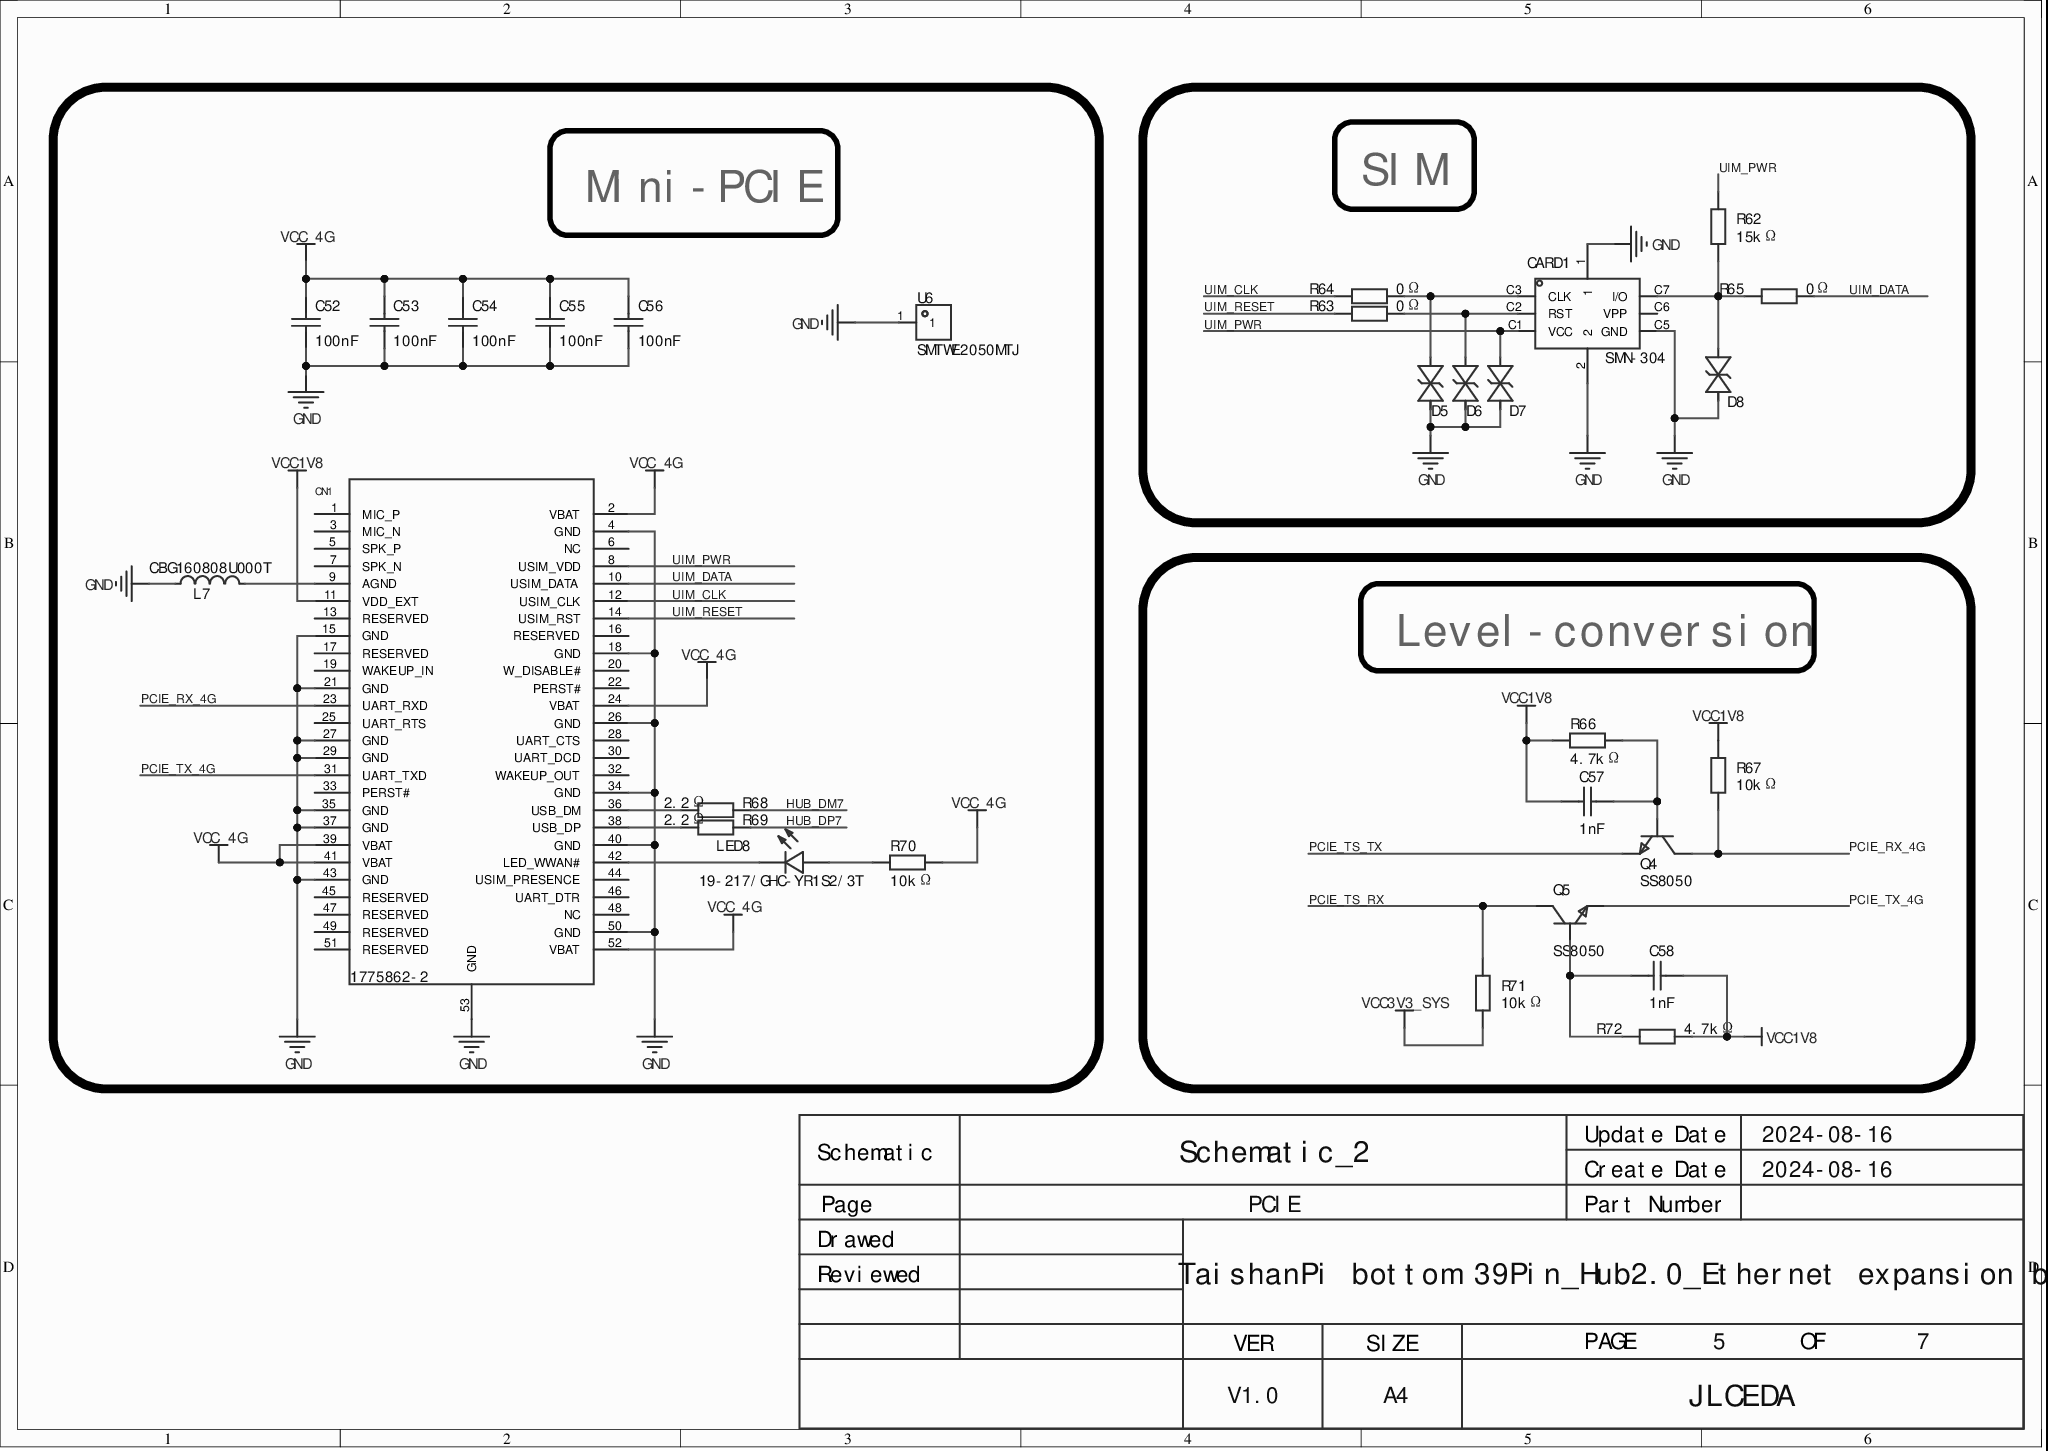
[diagram p0: MISC84334-6.SchDoc]
# Altium project MISC84334.PrjPcb (part 4 of 5)
## Sheet MISC84334-6.SchDoc (continued)
### Library data of the parts (continued)
R70 = 0402WGF1002TCE: Resistor type:Thick film resistor;Resistance:10kΩ;Tolerance:±1%;Power:62.5mW;Max working voltage:50V;Temp. coefficient:±100ppm/℃;; Manufacturer: UNI-ROYAL(厚声); Symbol: RC0402JR-07510RL; AddInBom: yes; ModelId: 671aefced39d4c318694bba8bd8efd39; ModelName: R0402_L1.0-W0.5-H0.5; ModelTransform: 39.37,19.685,0,0,0,0,0,0.0005,0; Tolerance: ±1%; Power(Watts): 62.5mW; Overload Voltage (Max): 50V; LCSC Part Name: 10kΩ ±1% 62.5mW 厚膜电阻; JLCPCB Part Class: Basic Part; Device: 0402WGF1002TCE; SupplierPart: C25744; ManufacturerPart: 0402WGF1002TCE; Supplier Footprint: 0402; Datasheet: https://atta.szlcsc.com/upload/public/pdf/source/20200306/C422600_1E6D84923E4A46A82E41ADD87F860B5C.pdf; Supplier: LCSC; ConvertToPcb: yes; FootprintName: R0402; Type: Thick film resistor; Value: 10kΩ; Temperature Coefficient: ±100ppm/℃; Operating Temperature Range: -55℃~+155℃
U6 = SMTWE2050MTJ: M2x4.35xL5+1.4; Symbol: SMTWE205MTJ; AddInBom: yes; ModelId: 49167c91e1ea4c02a5f8b62a6a5870e0; ModelTransform: 171.2595,171.17147,0,0,0,0,-0.002,0,-55.118; Supplier Part: C2928179; Device: SMTWE2050MTJ; Supplier: LCSC; Manufacturer Part: SMTWE2050MTJ; LCSC Part Name: 雄和远景，电路板表贴圆螺母柱，M2X5，铁镀锡; Supplier Footprint: -; Datasheet: https://atta.szlcsc.com/upload/public/pdf/source/20211223/4247FA230B3B7DF26F2B26B8CCB35E37.pdf; ConvertToPcb: yes; FootprintName: SMD_BD4.4-L4.4-D2.8; ModelName: SMD_BD4.4-L4.4-D2.8

## Sheet MISC84334-7.SchDoc
size 297 x 210 mm; Symbol: Sheet-Symbol_A4; Company: JLCEDA; Version: V1.0; Page Size: A4; @Project Name: TaishanPi bottom 4G_HUB2.0_ET100_HS expansion board; @Page Count: 7; @Update Date: 2024-08-16; @Create Date: 2024-08-16; @Schematic Name: Schematic; @Page No: 1; @Page Name: POWER; Device: Sheet-Symbol_A4; @Board Name: TaishanPi bottom 4G_HUB2.0_ET100_HS expansion board; @Create Time: 14:34:06; @Update Time: 14:34:22
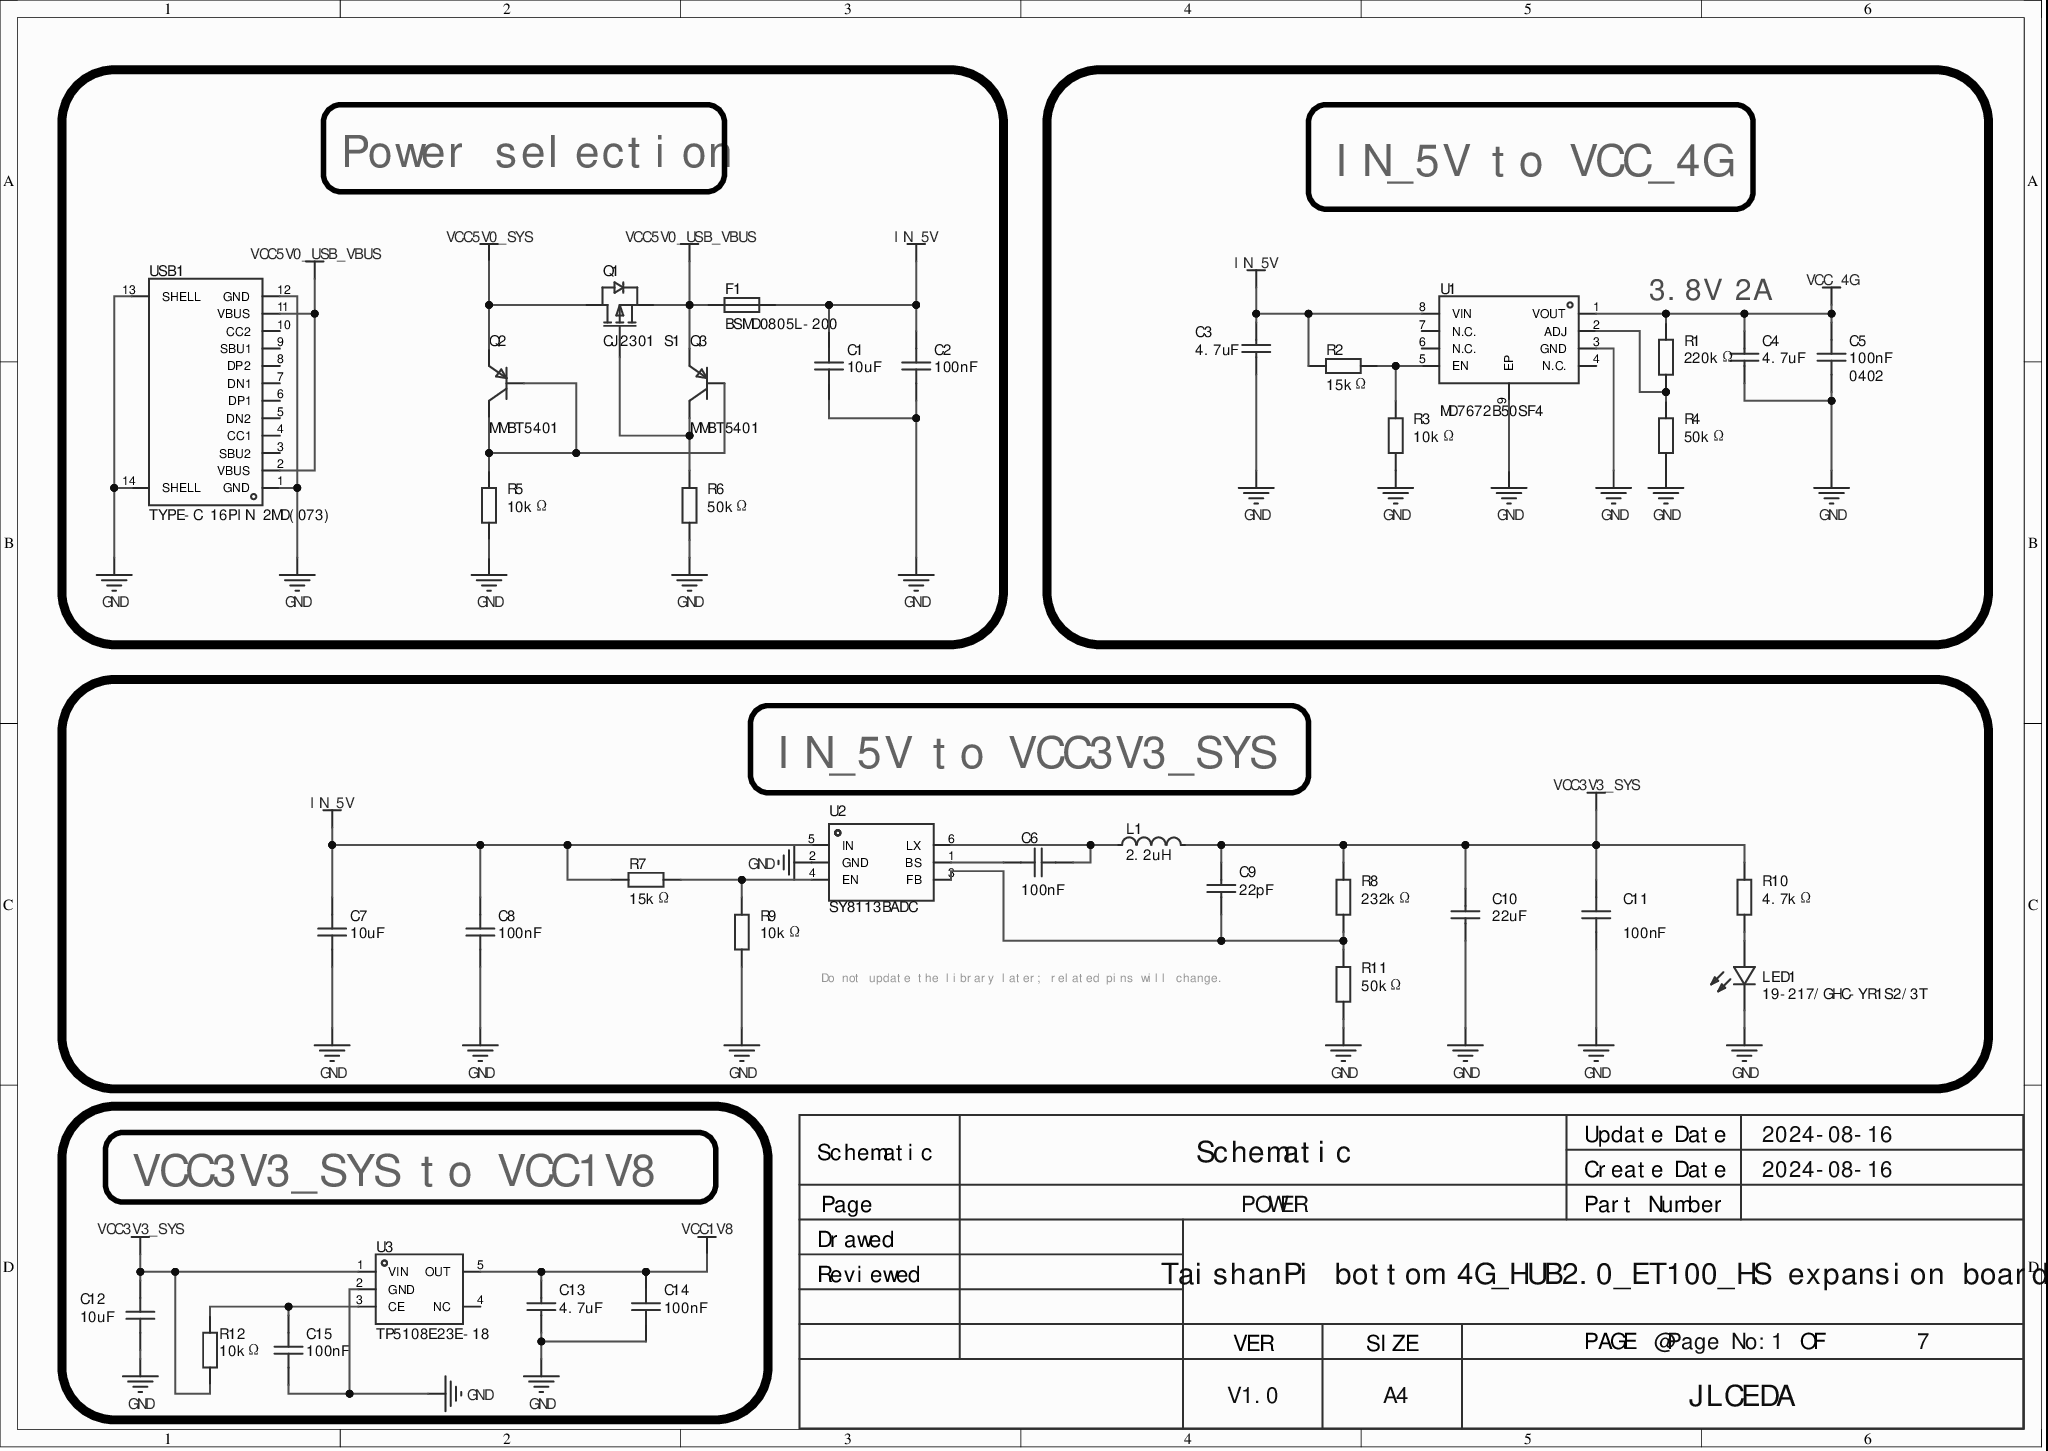
[diagram p1: MISC84334-7.SchDoc]

### Parts
C1  10uF  [r0603]
C2  100nF  [r0603]
C3  4.7uF  [C0603]
C4  4.7uF  [C0603]
C5  100nF  Supplier Footprint: 0402  [R0402]
C6  100nF  [R0402]
C7  10uF  [r0603]
C8  100nF  [r0603]
C9  22pF  [R0402]
C10  22uF  [r0603]
C11  100nF  [r0603]
C12  10uF  [r0603]
C13  4.7uF  [r0603]
C14  100nF  [C0603]
C15  100nF  [C0603]
F1  BSMD0805L-200  [F0805]
L1  2.2uH  [IND-SMD_L2.5-W2.0_WPN252012H]
LED1  19-217/GHC-YR1S2/3T  [LED0603-RD]
Q1  CJ2301 S1  [SOT-23-3_L3.0-W1.7-P0.95-LS2.9-BR]
Q2  MMBT5401  [SOT-23-3_L2.9-W1.3-P1.90-LS2.4-BR]
Q3  MMBT5401  [SOT-23-3_L2.9-W1.3-P1.90-LS2.4-BR]
R1  220kΩ  [R0402]
R2  15kΩ  [R0402]
R3  10kΩ  [R0402]
R4  50kΩ  [R0402]
R5  10kΩ  [R0402]
R6  50kΩ  [R0402]
R7  15kΩ  [R0402]
R8  232kΩ  [R0402]
R9  10kΩ  [R0402]
R10  4.7kΩ  [R0402]
R11  50kΩ  [R0402]
R12  10kΩ  [R0603]
U1  MD7672B50SF4  [ESOP-8_L4.9-W3.9-P1.27-LS6.0-BL-EP]
U2  SY8113BADC  [TSOT-23-6_L2.9-W1.6-P0.95-LS2.8-BR]
U3  TP5108E23E-18  [SOT-23-5_L3.0-W1.7-P0.95-LS2.8-BL]
USB1  TYPE-C 16PIN 2MD(073)  [USB-C-SMD_TYPE-C-6PIN-2MD-073]

### Blocks framed on the sheet
Power selection: C1 C2 F1 Q1-Q3 R5 R6 USB1
IN_5V to VCC_4G: C3-C5 R1-R4 U1
IN_5V to VCC3V3_SYS: C6-C11 L1 LED1 R7-R11 U2
VCC3V3_SYS to VCC1V8: C12-C15 R12 U3

### Nets
GND: C1.1 C2.1 C3.1 C4.1 C5.1 C7.1 C8.1 C10.1 C11.1 C12.1 C13.1 C14.1 C15.1 LED1.1(C) R3.1 R4.1 R5.1 R6.1 R9.1 R11.1 U1.3(GND) U1.9(EP) U2.2(GND) U3.2(GND) USB1.1(GND) USB1.12(GND) USB1.13(SHELL) USB1.14(SHELL)
IN_5V: C1.2 C2.2 C3.2 C7.2 C8.2 F1.2 R2.2 R7.2 U1.8(VIN) U2.5(IN)
VCC1V8: C13.2 C14.2 U3.5(OUT)
VCC3V3_SYS: C9.2 C10.2 C11.2 C12.2 L1.2 R8.2 R10.2 R12.1 U3.1(VIN)
VCC5V0_SYS: Q1.3(D) Q2.2(E)
VCC5V0_USB_VBUS: F1.1 Q1.2(S) Q3.2(E) USB1.2(VBUS) USB1.11(VBUS)
VCC_4G: C4.2 C5.2 R1.2 U1.1(VOUT)
NetC6_1: C6.1 L1.1 U2.6(LX)
NetC6_2: C6.2 U2.1(BS)
NetC9_1: C9.1 R8.1 R11.2 U2.3(FB)
NetC15_2: C15.2 R12.2 U3.3(CE)
NetLED1_2: LED1.2(A) R10.1
NetQ1_1: Q1.1(G) Q3.3(C) R6.2
NetQ2_1: Q2.1(B) Q2.3(C) Q3.1(B) R5.2
NetR1_1: R1.1 R4.2 U1.2(ADJ)
NetR2_1: R2.1 R3.2 U1.5(EN)
NetR7_1: R7.1 R9.2 U2.4(EN)

Not connected (* = marked no-connect by the designer): U1 4(N.C.)* 6(N.C.)* 7(N.C.)*; U3 4(NC)*; USB1 3(SBU2) 4(CC1) 5(DN2) 6(DP1) 7(DN1) 8(DP2) 9(SBU1) 10(CC2)

### Notes on the sheet
- 3.8V 2A
- Do not update the library later; related pins will change.
- Update Date
- 2024-08-16
- Schematic
- Page
- POWER
- Create Date
- Part Number
- Reviewed
- Drawed
- TaishanPi bottom 4G_HUB2.0_ET100_HS expansion board
- VER
- V1.0
- SIZE
- A4
- PAGE
- @Page No:1
- JLCEDA
- OF
- 7

### Library data of the parts
C1 = CL10A106KP8NNNC: Capacitance:10uF;Tolerance:±10%;Rated voltage:10V;Dielectric(Temp. coefficient):X5R;; Manufacturer: SAMSUNG(三星); AddInBom: yes; ModelId: ac125912035d415993ca9572d50418b1; ModelName: C0603_L1.6-W0.8-H0.8; ModelTransform: 62.992,31.496,0,0,0,0,0,0,0; Tolerance: ±10%; Voltage Rated: 10V; Temperature Coefficient: X5R; Supplier Footprint: 0603; Device: CL10A106KP8NNNC; Symbol: CL10A106KP8NNNC; LCSC Part Name: 10uF ±10% 10V; SupplierPart: C19702; ManufacturerPart: CL10A106KP8NNNC; JLCPCB Part Class: Basic Part; Datasheet: https://atta.szlcsc.com/upload/public/pdf/source/20160103/1457707703378.pdf; Supplier: LCSC; ConvertToPcb: yes; FootprintName: r0603; Value: 10uF
C2 C8 C11 C14 C15 = CC0603KRX7R9BB104: Capacitance:100nF;Tolerance:±10%;Rated voltage:50V;Dielectric(Temp. coefficient):X7R;; Manufacturer: YAGEO(国巨); AddInBom: yes; ModelId: ac125912035d415993ca9572d50418b1; ModelName: C0603_L1.6-W0.8-H0.8; ModelTransform: 62.992,31.496,0,0,0,0,0,0,0; Tolerance: ±10%; Voltage Rated: 50V; Temperature Coefficient: X7R; Device: CC0603KRX7R9BB104; Symbol: CC0603KRX7R9BB104; LCSC Part Name: 100nF ±10% 50V; SupplierPart: C14663; ManufacturerPart: CC0603KRX7R9BB104; Supplier Footprint: 0603; JLCPCB Part Class: Basic Part; Datasheet: https://atta.szlcsc.com/upload/public/pdf/source/20170116/1484561234239.pdf; Supplier: LCSC; ConvertToPcb: yes; Value: 100nF
  C2 C8 C11: FootprintName: r0603
  C14 C15: FootprintName: C0603
C3 C4 = CL10A475KP8NNNC: Capacitance:4.7uF;Tolerance:±10%;Rated voltage:10V;Dielectric(Temp. coefficient):X5R;; Manufacturer: SAMSUNG(三星); AddInBom: yes; ModelId: ac125912035d415993ca9572d50418b1; ModelName: C0603_L1.6-W0.8-H0.8; ModelTransform: 62.992,31.496,0,0,0,0,0,0,0; Tolerance: ±10%; Voltage Rated: 10V; Temperature Coefficient: X5R; Supplier Footprint: 0603; Device: CL10A475KP8NNNC; Symbol: CL10A475KP8NNNC; LCSC Part Name: 4.7uF ±10% 10V; SupplierPart: C1705; ManufacturerPart: CL10A475KP8NNNC; Datasheet: https://atta.szlcsc.com/upload/public/pdf/source/20160103/1457707692180.pdf; Supplier: LCSC; ConvertToPcb: yes; FootprintName: C0603; Value: 4.7uF
C5 = CC0402KRX7R7BB104: Capacitance:100nF;Tolerance:±10%;Rated voltage:16V;Dielectric(Temp. coefficient):X7R;; Manufacturer: YAGEO(国巨); AddInBom: yes; ModelId: 36a51122f27c49738f86b3bfa98863e0; ModelName: C0402_L1.0-W0.5-H0.5; ModelTransform: 39.37,19.685,0,0,0,0,0,0,0; Tolerance: ±10%; Voltage Rated: 16V; Temperature Coefficient: X7R; Device: CC0402KRX7R7BB104; Symbol: CC0402KRX7R7BB104; LCSC Part Name: 100nF ±10% 16V; SupplierPart: C60474; ManufacturerPart: CC0402KRX7R7BB104; Datasheet: https://atta.szlcsc.com/upload/public/pdf/source/20211223/9278FD768280B81DDBEF48FA36411A03.pdf; Supplier: LCSC; ConvertToPcb: yes; FootprintName: R0402; Value: 100nF
C6 = CL05B104KB54PNC: Capacitance:100nF;Tolerance:±10%;Rated voltage:50V;Dielectric(Temp. coefficient):X7R;; Manufacturer: SAMSUNG(三星); AddInBom: yes; ModelId: 36a51122f27c49738f86b3bfa98863e0; ModelName: C0402_L1.0-W0.5-H0.5; ModelTransform: 39.37,19.685,0,0,0,0,0,0,0; Tolerance: ±10%; Voltage Rated: 50V; Temperature Coefficient: X7R; Device: CL05B104KB54PNC; Symbol: CL05B104KB54PNC; LCSC Part Name: 100nF ±10% 50V; SupplierPart: C307331; ManufacturerPart: CL05B104KB54PNC; Supplier Footprint: 0402; JLCPCB Part Class: Basic library; Datasheet: https://atta.szlcsc.com/upload/public/pdf/source/20181009/C307331_222F7C870FD3EA5F46F538B483443886.pdf; Supplier: LCSC; ConvertToPcb: yes; FootprintName: R0402; Value: 100nF
C7 C12 = 0603X106M100CT: Capacitance:10uF;Tolerance:±20%;Rated voltage:10V;Dielectric(Temp. coefficient):X5R;; Manufacturer: Walsin(华新科); AddInBom: yes; ModelId: ac125912035d415993ca9572d50418b1; ModelName: C0603_L1.6-W0.8-H0.8; ModelTransform: 62.992,31.496,0,0,0,0,0,0,0; Tolerance: ±20%; Voltage Rated: 10V; Temperature Coefficient: X5R; Device: 0603X106M100CT; Symbol: 0603X106M100; LCSC Part Name: 10uF ±20% 10V; SupplierPart: C89283; ManufacturerPart: 0603X106M100CT; Supplier Footprint: 0603; JLCPCB Part Class: Extended library; Datasheet: https://atta.szlcsc.com/upload/public/pdf/source/20161226/1482720147964.pdf; Supplier: LCSC; ConvertToPcb: yes; FootprintName: r0603; Value: 10uF
C9 = 0402CG220J500NT: Capacitance:22pF;Tolerance:±5%;Rated voltage:50V;Dielectric(Temp. coefficient):C0G;; Manufacturer: FH(风华); AddInBom: yes; ModelId: 36a51122f27c49738f86b3bfa98863e0; ModelName: C0402_L1.0-W0.5-H0.5; ModelTransform: 39.37,19.685,0,0,0,0,0,0,0; Tolerance: ±5%; Voltage Rated: 50V; Temperature Coefficient: C0G; Device: 0402CG220J500NT; Symbol: 0402CG220J500NT; LCSC Part Name: 22pF ±5% 50V; SupplierPart: C1555; ManufacturerPart: 0402CG220J500NT; Supplier Footprint: 0402; JLCPCB Part Class: Basic Part; Datasheet: https://atta.szlcsc.com/upload/public/pdf/source/20170923/C1555_1506149269156988362.pdf; Supplier: LCSC; ConvertToPcb: yes; FootprintName: R0402; Value: 22pF
C10 = GRT188R61A226ME13D: Capacitance:22uF;Tolerance:±20%;Rated voltage:10V;Dielectric(Temp. coefficient):X5R;; Manufacturer: muRata(村田); AddInBom: yes; ModelId: ac125912035d415993ca9572d50418b1; ModelName: C0603_L1.6-W0.8-H0.8; ModelTransform: 62.992,31.496,0,0,0,0,0,0,0; Tolerance: ±20%; Voltage Rated: 10V; Temperature Coefficient: X5R; Device: GRT188R61A226ME13D; Symbol: GRT188R61A226ME13D; LCSC Part Name: 22uF ±20% 10V; SupplierPart: C126630; ManufacturerPart: GRT188R61A226ME13D; Supplier Footprint: 0603; JLCPCB Part Class: Extended library; Datasheet: https://atta.szlcsc.com/upload/public/pdf/source/20180326/C126630_30AAFCB8DD5A84EA71B92B07E45A02B6.pdf; Supplier: LCSC; ConvertToPcb: yes; FootprintName: r0603; Value: 22uF
C13 = CL10A475KO8NNNC: Capacitance:4.7uF;Tolerance:±10%;Rated voltage:16V;Dielectric(Temp. coefficient):X5R;; Manufacturer: SAMSUNG(三星); AddInBom: yes; ModelId: ac125912035d415993ca9572d50418b1; ModelName: C0603_L1.6-W0.8-H0.8; ModelTransform: 62.992,31.496,0,0,0,0,0,0,0; Tolerance: ±10%; Voltage Rated: 16V; Temperature Coefficient: X5R; Device: CL10A475KO8NNNC; Symbol: CL10A475KO8NNNC; LCSC Part Name: 4.7uF ±10% 16V; SupplierPart: C19666; ManufacturerPart: CL10A475KO8NNNC; Supplier Footprint: 0603; JLCPCB Part Class: Basic Part; Datasheet: https://atta.szlcsc.com/upload/public/pdf/source/20160103/1457707703134.pdf; Supplier: LCSC; ConvertToPcb: yes; FootprintName: r0603; Value: 4.7uF
F1 = BSMD0805L-200: Max voltage:6V;Max current:50A;Hold current:2A;Trip current:4A;; Manufacturer: BHFUSE(佰宏); AddInBom: yes; ModelId: 57e2aa106f9143e8b6ab832aebb31c78; ModelName: F0805_L2.1-W1.4-H0.8; ModelTransform: 82.677,55.118,0,0,0,0,0.0005,0,0; Operating Voltage (Max): 6V; Current Rating (Max): 50A; Hold Current: 2A; Trip Current: 4A; Power Dissipation: 1W; Resistance - Initial (Ri) (Min): 4mΩ; Resistance - Post Trip (R1) (Max): 45mΩ; Maximum Time to Trip: 5s; Device: BSMD0805L-200; Symbol: BSMD0805L-200; LCSC Part Name: 6V 2A 0805自恢复 5秒内动作; SupplierPart: C2757931; ManufacturerPart: BSMD0805L-200; Supplier Footprint: 0805; Datasheet: https://atta.szlcsc.com/upload/public/pdf/source/20220302/84A1D93E6CA84F7719C829CBF191FAF8.pdf; Supplier: LCSC; ConvertToPcb: yes; FootprintName: F0805; Operating Temperature: -40℃~+85℃
L1 = WPN252012H2R2MT: Type:-;Inductance:2.2uH;Tolerance:±20%;Rated current:1.9A;Saturation current(Isat):3A;; Manufacturer: Sunlord(顺络); Symbol: SWPA4030S4R7MT; AddInBom: yes; ModelId: 7ae8e774cfcf498ea5119a488d0de531; ModelName: IND-SMD_L2.5-W2.0-H1.2-252012; ModelTransform: 78.74,99.2124,0,90,0,0,0,0,0; Tolerance: ±20%; Rated Current: 1.9A; Saturation Current (Isat): 3A; DC Resistance (DCR): 120mΩ; Height: 3mm; Width: 4mm; Length: 4mm; Device: WPN252012H2R2MT; LCSC Part Name: 2.2uH ±20% 3A; SupplierPart: C98350; ManufacturerPart: WPN252012H2R2MT; Supplier Footprint: SMD; JLCPCB Part Class: Extended Part; Datasheet: https://atta.szlcsc.com/upload/public/pdf/source/20210916/5D33DED32780FEB7D0AA8BED8FC93477.pdf; Supplier: LCSC; ConvertToPcb: yes; FootprintName: IND-SMD_L2.5-W2.0_WPN252012H; Type: -; Value: 2.2uH; Ratings: -
LED1 = 19-217/GHC-YR1S2/3T: as LED8 on sheet MISC84334-6; Device: 19-217/GHC-YR1S2/3T; Symbol: 19-217/GHC-YR1S2/3T; LCSC Part Name: 19-217/GHC-YR1S2/3T; SupplierPart: C72043; ManufacturerPart: 19-217/GHC-YR1S2/3T; Supplier Footprint: 0603; JLCPCB Part Class: Basic Part; Datasheet: https://atta.szlcsc.com/upload/public/pdf/source/20160507/1462613613780.pdf; Supplier: LCSC; ConvertToPcb: yes; FootprintName: LED0603-RD; ModelName: LED0603-RD; Emitted Color: Emerald green; Diode Configuration: -; Dominant Wavelength: 520nm~535nm; Color Temperature: -; Mounting Sytle: -; Operating Temperature: -40℃~+85℃
Q1 = CJ2301 S1: Type:P-channel;drain-source voltage(Vdss):20V;continuous drain current(Id):2.3A;Power(Pd):350mW;on-resistance(RDS(on)@Vgs,Id):112mΩ@4.5V,2.8A;; Manufacturer: CJ(江苏长电/长晶); AddInBom: yes; ModelId: 89cb27a44ab2466697082bb9fd73a7d0; ModelName: SOT-23-3L_L2.9-W1.6-H1.1-LS2.8-P0.95; ModelTransform: 110.59301,114.173,0,180,0,0,0,-0.0005,0; Drain Source Voltage (Vdss): 20V; Continuous Drain Current (Id): 2.3A; Power Dissipation (Pd): 350mW; Gate Threshold Voltage (Vgs(th)@Id): 1V@250uA; Device: CJ2301 S1; Symbol: CJ2301 S1; LCSC Part Name: P沟道 20V 2.3A; SupplierPart: C8547; ManufacturerPart: CJ2301 S1; Supplier Footprint: SOT-23; JLCPCB Part Class: Extended library; Datasheet: https://atta.szlcsc.com/upload/public/pdf/source/20140815/1457707224119.pdf; Supplier: LCSC; ConvertToPcb: yes; FootprintName: SOT-23-3_L3.0-W1.7-P0.95-LS2.9-BR; Type: P-channel; Drain Source On Resistance (RDS(on)@Vgs,Id): 112mΩ@4.5V,2.8A; Total Gate Charge (Qg@Vgs): -; Input Capacitance (Ciss@Vds): -; Reverse Transfer Capacitance (Crss@Vds): -
Q2 Q3 = MMBT5401_C8326: Transistor type:PNP;Vce breakdown voltage(Vceo):150V;collector current(Ic):600mA;Power(Pd):300mW;collector cutoff current(Icbo):100nA;Vce saturation voltage(VCE(sat)@Ic,Ib):500mV@50mA,5mA;DC current gain(hFE@Ic,Vce):200@10mA,5V;transition frequency(fT):100MHz;Operating temperature:+150℃@(Tj);; Manufacturer: CJ(江苏长电/长晶); AddInBom: yes; ModelId: c62791f0466c4ae2a892c056b845b0ca; ModelName: SOT-23-3P_L2.9-W1.3-H1.0-LS2.4-P0.95; ModelTransform: 98.425,114.173,0,180,0,0,0.0005,-0.0005,0; Transistor Type: PNP; Collector-Emitter Breakdown Voltage (Vceo): 150V; Collector Current (Ic): 600mA; Power Dissipation (Pd): 300mW; Collector Cut-Off Current (Icbo): 100nA; Transition Frequency (fT): 100MHz; Device: MMBT5401_C8326; Symbol: MMBT5401; LCSC Part Name: PNP 150V 600mA; SupplierPart: C8326; ManufacturerPart: MMBT5401; Supplier Footprint: SOT-23; Datasheet: https://atta.szlcsc.com/upload/public/pdf/source/20140809/1457707213644.pdf; Supplier: LCSC; ConvertToPcb: yes; FootprintName: SOT-23-3_L2.9-W1.3-P1.90-LS2.4-BR; Collector-Emitter Saturation Voltage (VCE(sat)@Ic,Ib): 500mV@50mA,5mA; DC Current Gain (hFE@Ic,Vce): 200@10mA,5V; Operating Temperature: +150℃@(Tj)
R1 = 0402WGF2203TCE: Resistor type:Thick film resistor;Resistance:220kΩ;Tolerance:±1%;Power:62.5mW;; Manufacturer: UNI-ROYAL(厚声); AddInBom: yes; ModelId: 671aefced39d4c318694bba8bd8efd39; ModelName: R0402_L1.0-W0.5-H0.5; ModelTransform: 39.37,19.685,0,0,0,0,0,0.0005,0; Tolerance: ±1%; Power(Watts): 62.5mW; Temperature Coefficient: ±100ppm/℃; Overload Voltage (Max): 50V; Device: 0402WGF2203TCE; Symbol: 0402WGF2203TCE; LCSC Part Name: 220kΩ ±1% 62.5mW; SupplierPart: C25767; ManufacturerPart: 0402WGF2203TCE; Supplier Footprint: 0402; Datasheet: https://atta.szlcsc.com/upload/public/pdf/source/20200306/C422600_1E6D84923E4A46A82E41ADD87F860B5C.pdf; Supplier: LCSC; ConvertToPcb: yes; FootprintName: R0402; Type: Thick film resistor; Value: 220kΩ; Operating Temperature Range: -55℃~+155℃
R2 R7 = 0402WGF1502TCE: as R62 on sheet MISC84334-6; Supplier Footprint: 0402; Device: 0402WGF1502TCE; Symbol: 0402WGF1502TCE; LCSC Part Name: 15kΩ ±1% 62.5mW; SupplierPart: C25756; ManufacturerPart: 0402WGF1502TCE; JLCPCB Part Class: Basic library; Datasheet: https://atta.szlcsc.com/upload/public/pdf/source/20200306/C422600_1E6D84923E4A46A82E41ADD87F860B5C.pdf; Supplier: LCSC; ConvertToPcb: yes; FootprintName: R0402; Type: Thick film resistor; Value: 15kΩ; Operating Temperature Range: -55℃~+155℃
R3 R5 R9 = 0402WGF1002TCE: as R67 on sheet MISC84334-6; Symbol: 0402WGF1002TCE; Device: 0402WGF1002TCE; Supplier: LCSC; Manufacturer Part: 0402WGF1002TCE; Supplier Part: C25744; Value: 10kΩ; JLCPCB Part Class: Basic library; LCSC Part Name: 10kΩ ±1% 62.5mW; Supplier Footprint: 0402; Datasheet: https://atta.szlcsc.com/upload/public/pdf/source/20200306/C422600_1E6D84923E4A46A82E41ADD87F860B5C.pdf; ConvertToPcb: yes; FootprintName: R0402; Type: Thick film resistor; Operating Temperature Range: -55℃~+155℃
R4 R6 R11 = RTT025002FTH: Resistor type:Thick film resistor;Resistance:50kΩ;Tolerance:±1%;Power:62.5mW;; Manufacturer: RALEC(旺诠); AddInBom: yes; ModelId: 671aefced39d4c318694bba8bd8efd39; ModelName: R0402_L1.0-W0.5-H0.5; ModelTransform: 39.37,19.685,0,0,0,0,0,0.0005,0; Tolerance: ±1%; Power(Watts): 62.5mW; Temperature Coefficient: ±100ppm/℃; Overload Voltage (Max): 50V; Device: RTT025002FTH; Symbol: RTT025002FTH; LCSC Part Name: 50kΩ ±1% 62.5mW; SupplierPart: C166559; ManufacturerPart: RTT025002FTH; Supplier Footprint: 0402; JLCPCB Part Class: Extended library; Datasheet: https://atta.szlcsc.com/upload/public/pdf/source/20180202/C166559_15175647488101336234.pdf; Supplier: LCSC; ConvertToPcb: yes; FootprintName: R0402; Type: Thick film resistor; Value: 50kΩ; Operating Temperature Range: -55℃~+155℃
R8 = 0402WGF2323TCE: Resistor type:Thick film resistor;Resistance:232kΩ;Tolerance:±1%;Power:62.5mW;Temp. coefficient:±100ppm/℃;Max working voltage:50V;Operating temperature:-55℃~+155℃;; Manufacturer: UNI-ROYAL(厚声); AddInBom: yes; ModelId: 671aefced39d4c318694bba8bd8efd39; ModelName: R0402_L1.0-W0.5-H0.5; ModelTransform: 39.37,19.685,0,0,0,0,0,0.0005,0; Tolerance: ±1%; Power(Watts): 62.5mW; Overload Voltage (Max): 50V; LCSC Part Name: 232kΩ ±1% 62.5mW; JLCPCB Part Class: Extended Part; Device: 0402WGF2323TCE; Symbol: 0402WGF2323TCE; SupplierPart: C27000; ManufacturerPart: 0402WGF2323TCE; Supplier Footprint: 0402; Datasheet: https://atta.szlcsc.com/upload/public/pdf/source/20200306/C422600_1E6D84923E4A46A82E41ADD87F860B5C.pdf; Supplier: LCSC; ConvertToPcb: yes; FootprintName: R0402; Type: Thick film resistor; Value: 232kΩ; Temperature Coefficient: ±100ppm/℃; Operating Temperature Range: -55℃~+155℃
R10 = 0402WGF4701TCE: as R66 on sheet MISC84334-6; Symbol: 0402WGF4701TCE; Device: 0402WGF4701TCE; Supplier: LCSC; Manufacturer Part: 0402WGF4701TCE; Supplier Part: C25900; Value: 4.7kΩ; JLCPCB Part Class: Basic library; LCSC Part Name: 4.7kΩ ±1% 62.5mW; Supplier Footprint: 0402; Datasheet: https://atta.szlcsc.com/upload/public/pdf/source/20200306/C422600_1E6D84923E4A46A82E41ADD87F860B5C.pdf; ConvertToPcb: yes; FootprintName: R0402; Type: Thick film resistor; Operating Temperature Range: -55℃~+155℃
R12 = 0603WAF1002T5E: Resistor type:Thick film resistor;Resistance:10kΩ;Tolerance:±1%;Power:100mW;; Manufacturer: UNI-ROYAL(厚声); AddInBom: yes; ModelId: fc143cca1e79419f9cd78b61e9279f08; ModelTransform: 31.8897,63.7794,0,90,0,0,0,0,0; Tolerance: ±1%; Power(Watts): 100mW; Temperature Coefficient: ±100ppm/℃; Overload Voltage (Max): 75V; Device: 0603WAF1002T5E; Symbol: 0603WAF1002T5E; LCSC Part Name: 厚膜电阻 10kΩ ±1% 100mW; SupplierPart: C25804; ManufacturerPart: 0603WAF1002T5E; Supplier Footprint: 0603; JLCPCB Part Class: Basic library; Datasheet: https://atta.szlcsc.com/upload/public/pdf/source/20200306/C422600_1E6D84923E4A46A82E41ADD87F860B5C.pdf; Supplier: LCSC; ConvertToPcb: yes; FootprintName: R0603; ModelName: R0603; Type: Thick film resistor; Value: 10kΩ; Operating Temperature Range: -55℃~+155℃
U1 = MD7672B50SF4: Output type:Adjustable;Output polarity:Positive;Max input voltage:6V;Output voltage:1.2V~5V;Output current:2A;; Manufacturer: 明达微; AddInBom: yes; ModelId: d3e00daa36c445139c055a3b9efb85d2; ModelName: ESOP-8_L4.9-W3.9-H1.6-LS6.0-P1.27; ModelTransform: 240.157,192.913,0,90,0,0,0,0,0; Number of Outputs: 1; Maximum Input Voltage: 6V; Output Current: 2A; Device: MD7672B50SF4; Symbol: MD7672B50SF4; LCSC Part Name: MD7672B50SF4; SupplierPart: C920526; ManufacturerPart: MD7672B50SF4; Supplier Footprint: SOP-8-EP; JLCPCB Part Class: Extended library; Datasheet: https://atta.szlcsc.com/upload/public/pdf/source/20201124/C920526_808F7D787368D9A2653AA854DB6B391C.pdf; Supplier: LCSC; ConvertToPcb: yes; FootprintName: ESOP-8_L4.9-W3.9-P1.27-LS6.0-BL-EP; Output Type: Adjustable; Output Polarity: Positive; Output Voltage: 1.2V~5V
U2 = SY8113BADC: Function type:Buck;Synchronous rectification:-;Output channels:-;Topology:-;Input voltage:-;Output current (max):-;Switching frequency:-;; Manufacturer: silergy(矽力杰); AddInBom: yes; Function: Buck; ModelId: 2c4039b5b88644c1bda4b4ba9e971667; ModelName: TSOT-23-6_L2.9-W1.6-H1.1-LS2.8-P0.95; ModelTransform: 110.45568,114.173,0,180,0,0,-0.005,-0.0005,0; JLCPCB Part Class: Extended Part; Device: SY8113BADC; LCSC Part Name: 降压型; SupplierPart: C78989; ManufacturerPart: SY8113BADC; Supplier Footprint: TSOT-23-6; Datasheet: https://atta.szlcsc.com/upload/public/pdf/source/20161125/1480067827505.pdf; Supplier: LCSC; ConvertToPcb: yes; Synchronous Rectification: -; Number of Outputs: -; Topology: -; Input Voltage: -; Output Current (Max): -; Switching Frequency: -; SymbolName: SY8113BADC; FootprintName: TSOT-23-6_L2.9-W1.6-P0.95-LS2.8-BR
U3 = TP5108E23E-18: Output type:-;; Manufacturer: TECH PUBLIC(台舟); AddInBom: yes; ModelId: 0a2a1b8f50944f73965918ad6e5fe167; ModelName: SOT-23-5_L2.9-W1.6-H1.1-LS2.8-P0.95; ModelTransform: 118.60433,114.173,0,90,0,0,0.0005,0.0005,0; Device: TP5108E23E-18; Symbol: TP5108E23E-18; LCSC Part Name: TP5108E23E-18; SupplierPart: C907845; ManufacturerPart: TP5108E23E-18; Supplier Footprint: SOT-23-5; JLCPCB Part Class: Extended Part; Datasheet: https://atta.szlcsc.com/upload/public/pdf/source/20210810/AA08377C81F8353E2F8C5F8FC160FE00.pdf; Supplier: LCSC; ConvertToPcb: yes; FootprintName: SOT-23-5_L3.0-W1.7-P0.95-LS2.8-BL; Output Type: -
USB1 = TYPE-C 16PIN 2MD(073): Connector type:Type-C;Standard:-;Gender:Female;Contacts:16P;Ports:1;Mounting:Horizontal SMD;Rated current - power:5A;Operating temperature:-25℃~+85℃;; Manufacturer: SHOU HAN(首韩); AddInBom: yes; ModelId: 3a41b9ec9b654a0fad4d118405ec6290; ModelTransform: 351.9678,298.4246,0,0,0,0,0,-47.244,-35.433; Gender: Female; Number of Contacts: 16P; Number of Ports: 1; Current Rating - Power (Max): 5A; Symbol: TYPE-C 16PIN 2MD(073); Device: TYPE-C 16PIN 2MD(073); Supplier: LCSC; Supplier Part: C2765186; Manufacturer Part: TYPE-C 16PIN 2MD(073); LCSC Part Name: Type-C 母 卧贴 带定位柱 不锈钢外壳 2次模顶; Supplier Footprint: SMD; Datasheet: https://atta.szlcsc.com/upload/public/pdf/source/20211123/39B17C16241EAC15C5E277BDA434118E.pdf; ConvertToPcb: yes; FootprintName: USB-C-SMD_TYPE-C-6PIN-2MD-073; ModelName: USB-C-SMD_TYPE-C-6PIN-2MD-073; Connector Type: Type-C; Standard: -; Mounting Style: Horizontal SMD; Operating Temperature Range: -25℃~+85℃